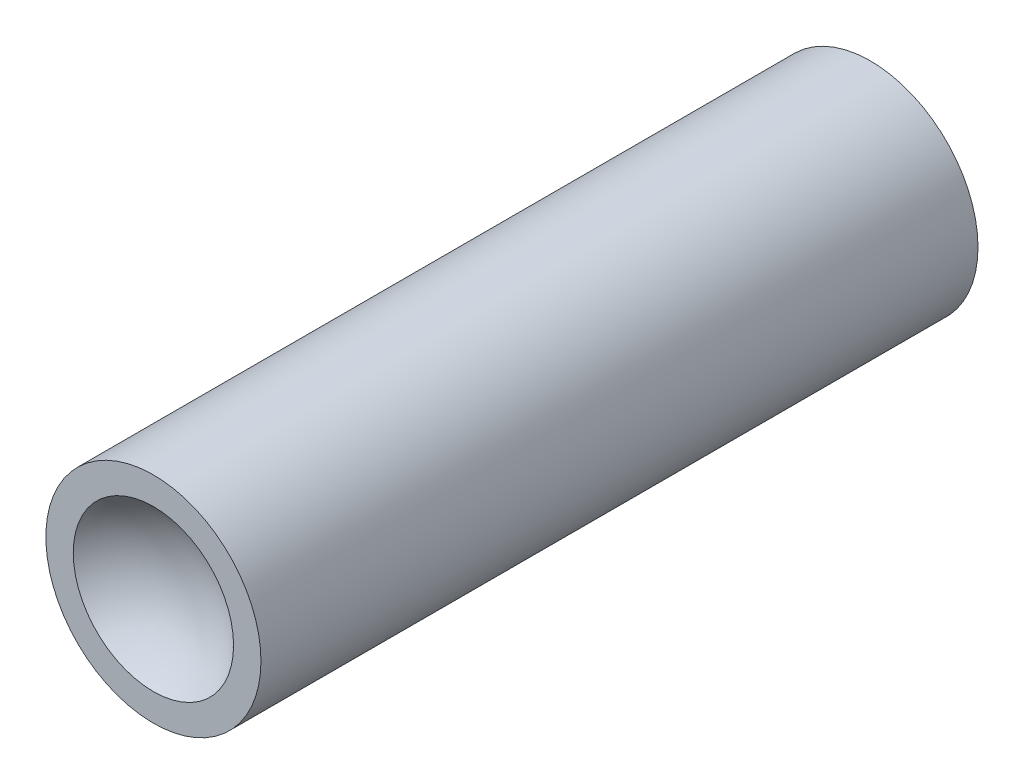
SolidWorks part; units mm, degrees
material "镀铬棒（硬）"
ref_plane "前视基准面" through (0, 0, 0) normal (0, 0, 1) x (1, 0, 0)
ref_plane "上视基准面" through (0, 0, 0) normal (0, 1, 0) x (1, 0, 0)
ref_plane "右视基准面" through (0, 0, 0) normal (1, 0, 0) x (0, 0, -1)
sketch "草图1" plane through (0, 0, 0) normal (0, 0, 1) x (1, 0, 0)
  circle A0 centre (0, 0) radius 6
  dimension "D1" = 12
extrude "凸台-拉伸1" add sketch "草图1" along normal blind 40
sketch "草图2" plane through (0, 0, 0) normal (0, 1, 0) x (1, 0, 0)
  line L0 (0, -44) -> (0, -40) construction
  line L1 (-6, -40) -> (6, -40) construction
  line L2 (0, -50) -> (0, -38) construction
  line L3 (0, -50) -> (0, -38)
  arc A0 (0, -38) -> (0, -50) centre (0, -44) ccw
  dimension "D1" = 12
  dimension "D2" = 4
revolve "切除-旋转4" cut sketch "草图2" angle 360 about L3
